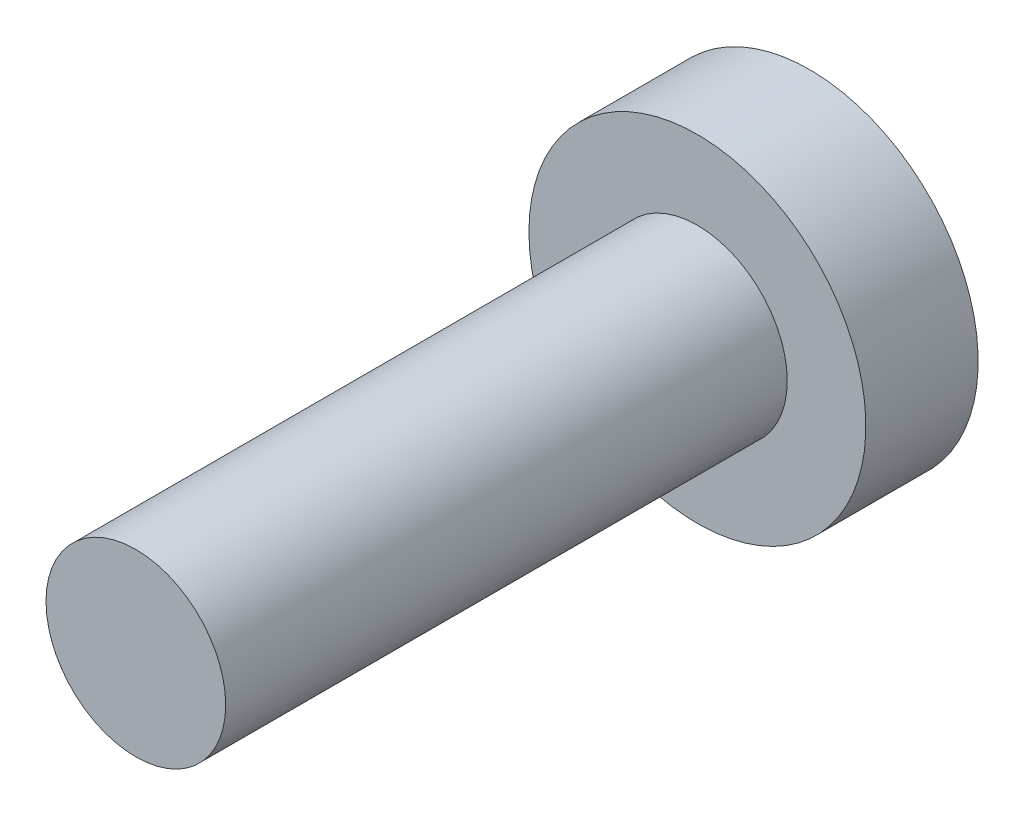
from build123d import *

# Parameters (mm, degrees)
SKETCH1_R           = 4
BOSS_EXTRUDE1_DEPTH = 25
SKETCH2_R           = 7.5
BOSS_EXTRUDE2_DEPTH = 5


with BuildPart() as part:
    # Sketch1 → Boss-Extrude1 (new body)
    with BuildSketch(Plane.XY):
        Circle(SKETCH1_R)
    extrude(amount=BOSS_EXTRUDE1_DEPTH)

    # Sketch2 → Boss-Extrude2 (add)
    with BuildSketch(Plane(origin=(0, 0, 0), x_dir=(-1, 0, 0), z_dir=(0, 0, -1))):
        Circle(SKETCH2_R)
    extrude(amount=BOSS_EXTRUDE2_DEPTH)


solid = part.part
